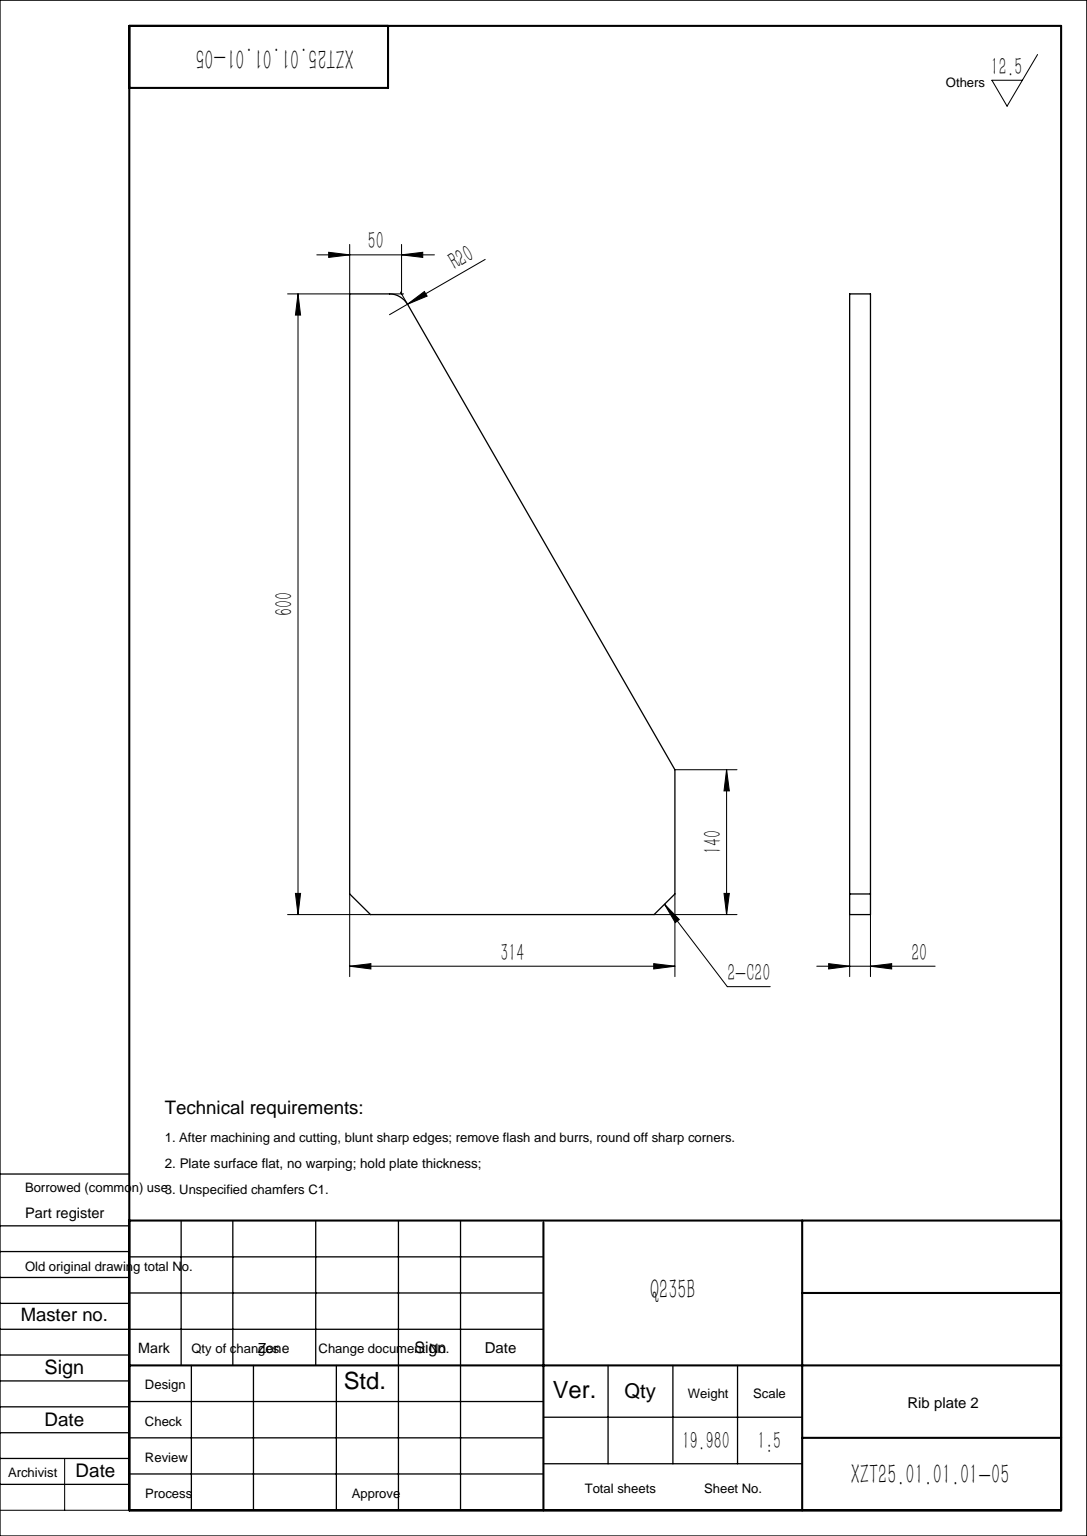
from build123d import *

# Parameters (mm, degrees)
BOSS_EXTRUDE1_DEPTH = 10
FILLET1_R           = 20
CHAMFER1_SIZE       = 20


with BuildPart() as part:
    # Sketch1 → Boss-Extrude1 (new, symmetric)
    with BuildSketch(Plane.XY):
        Polygon((0, 0), (314, 0), (314, 140), (50, 600), (0, 600), align=None)
    extrude(amount=BOSS_EXTRUDE1_DEPTH, both=True)

    # Fillet1
    fillet1_edges = [part.edges().sort_by_distance(p)[0] for p in [
        (50, 600, 0),
    ]]
    fillet(fillet1_edges, radius=FILLET1_R)

    # Chamfer1
    chamfer1_edges = [part.edges().sort_by_distance(p)[0] for p in [
        (314, 0, 0),
        (0, 0, 0),
    ]]
    chamfer(chamfer1_edges, length=CHAMFER1_SIZE)


solid = part.part
